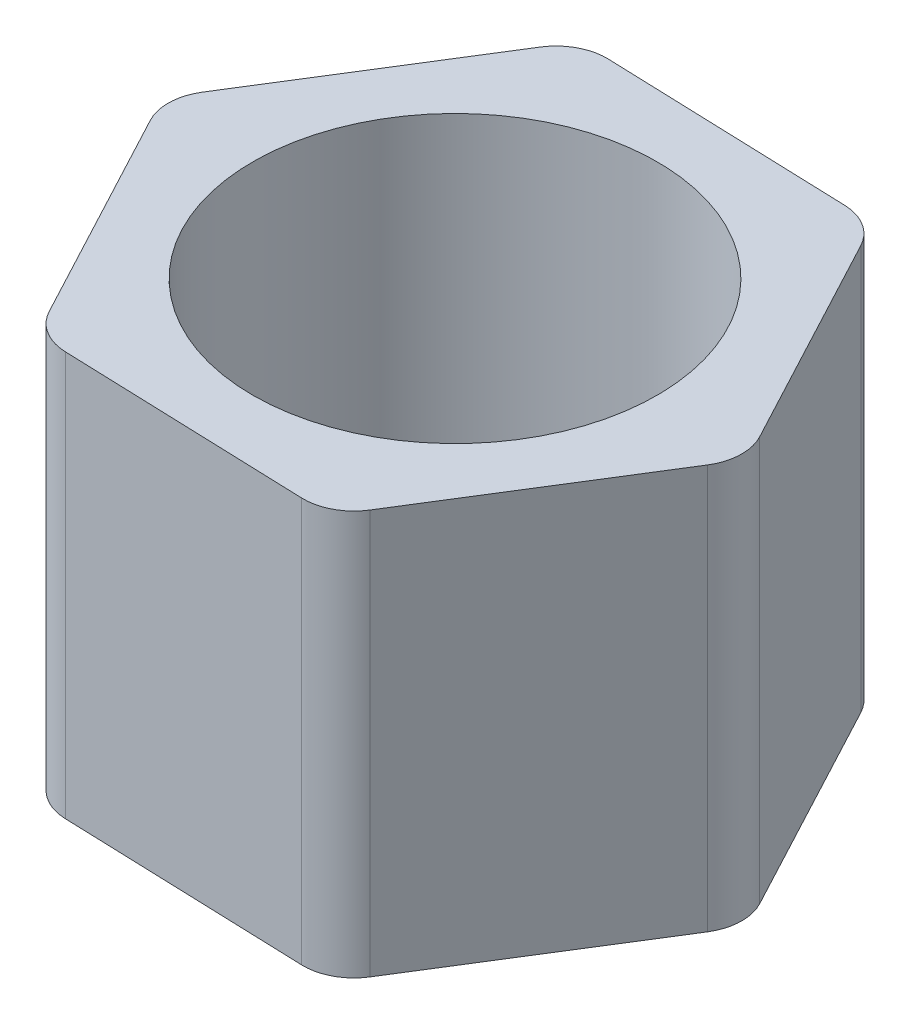
SolidWorks part; units mm, degrees
ref_plane "Front Plane" through (0, 0, 0) normal (0, 0, 1) x (1, 0, 0)
ref_plane "Top Plane" through (0, 0, 0) normal (0, 1, 0) x (1, 0, 0)
ref_plane "Right Plane" through (0, 0, 0) normal (1, 0, 0) x (0, 0, -1)
sketch "Sketch1" plane through (0, 0, 0) normal (0, 1, 0) x (1, 0, 0)
  line L1 (5.637, -10.5936) -> (11.9928, -0.415)
  line L2 (11.9928, -0.415) -> (6.3559, 10.1786)
  line L3 (6.3559, 10.1786) -> (-5.637, 10.5936)
  line L4 (-5.637, 10.5936) -> (-11.9928, 0.415)
  line L5 (-11.9928, 0.415) -> (-6.3559, -10.1786)
  line L6 (-6.3559, -10.1786) -> (5.637, -10.5936)
  circle A0 centre (0, 0) radius 12 construction
  circle A1 centre (0, 0) radius 8
extrude "Boss-Extrude1" add sketch "Sketch1" along normal blind 16
fillet "Fillet1" radius 2 1 edges at (5.637, 8, 10.5936)
fillet "Fillet2" radius 2 5 edges at (-5.637, 8, -10.5936) (-11.9928, 8, -0.415) (-6.3559, 8, 10.1786) (6.3559, 8, -10.1786) (11.9928, 8, 0.415)
